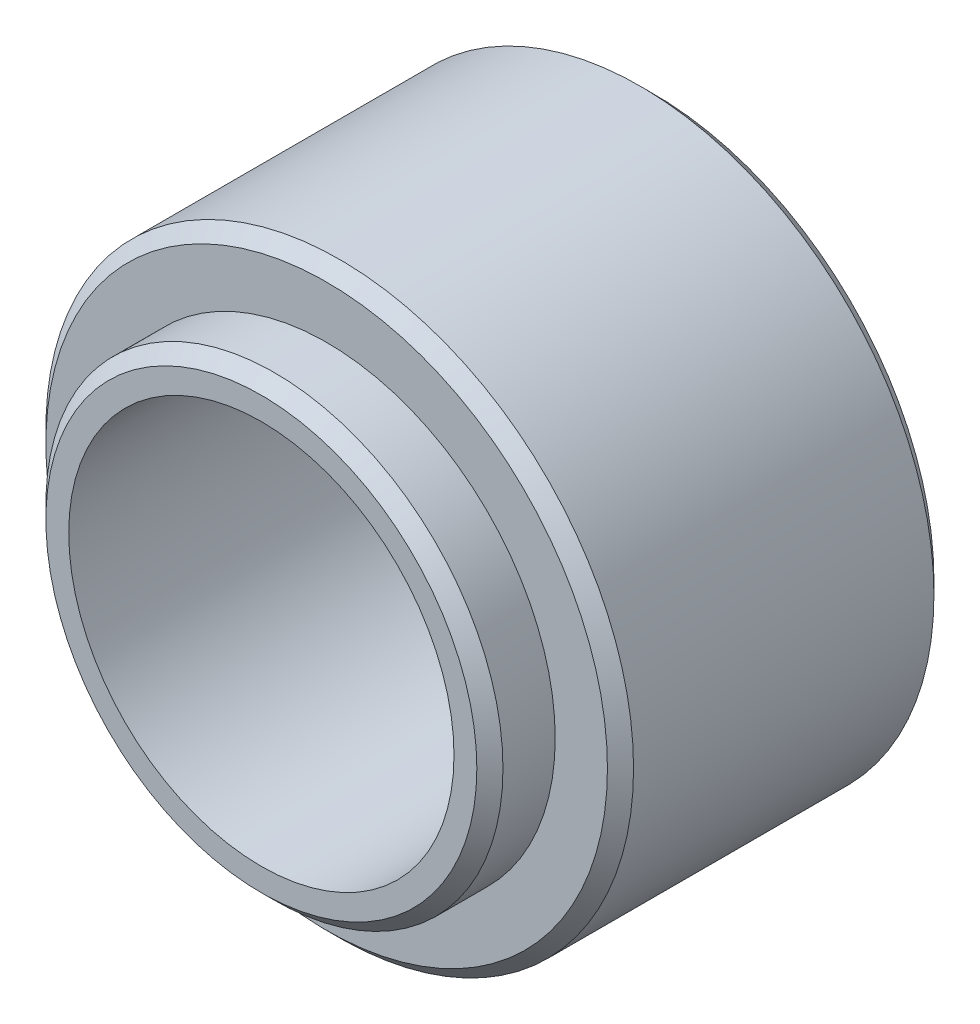
SolidWorks part; units mm, degrees
material "Plain carbon steel"
ref_plane "Front Plane" through (0, 0, 0) normal (0, 0, 1) x (1, 0, 0)
ref_plane "Top Plane" through (0, 0, 0) normal (0, 1, 0) x (1, 0, 0)
ref_plane "Right Plane" through (0, 0, 0) normal (1, 0, 0) x (0, 0, -1)
sketch "Sketch1" plane through (0, 0, 0) normal (0, 0, 1) x (1, 0, 0)
  circle A0 centre (0, 0) radius 22.5
  circle A1 centre (0, 0) radius 14.75
extrude "Boss-Extrude1" add sketch "Sketch1" along normal blind 25
sketch "Sketch2" plane through (0, 0, 25) normal (0, 0, 1) x (1, 0, 0)
  circle A0 centre (0, 0) radius 17.5
  circle A1 centre (0, 0) radius 14.75
extrude "Boss-Extrude2" add sketch "Sketch2" along normal blind 5
chamfer "Chamfer2" distance 1 distance2 1 3 edges at (22.5, 0, 0) (22.5, 0, 25) (17.5, 0, 30)
